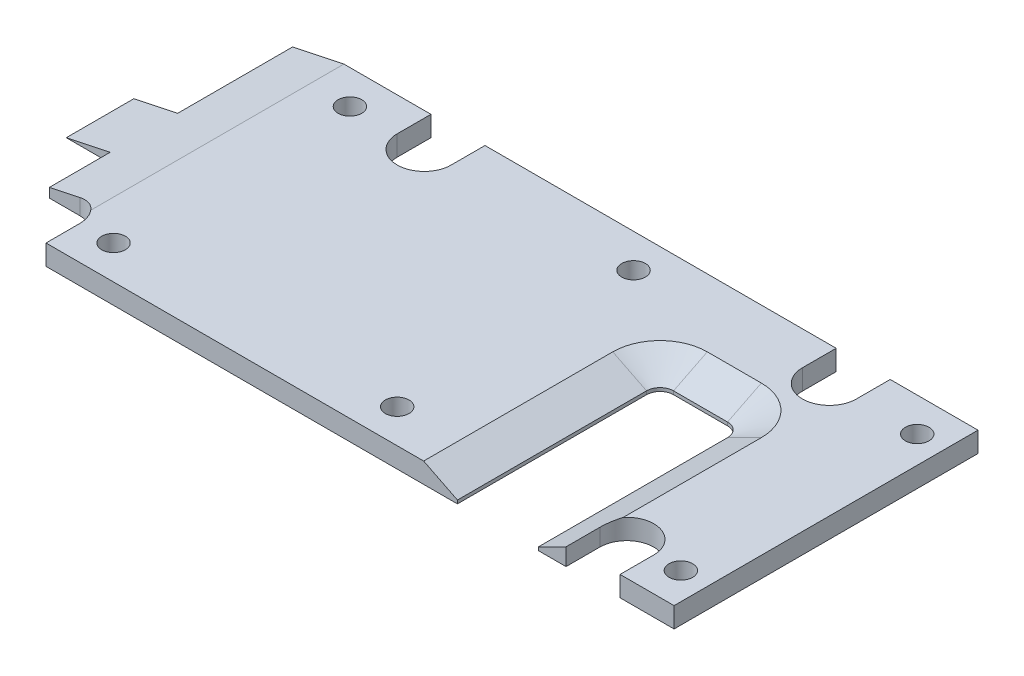
from build123d import *

# Parameters (mm, degrees)
SKETCH1_W           = 104.5
SKETCH1_H           = 45
BOSS_EXTRUDE1_DEPTH = 3
SKETCH2_W           = 12
SKETCH2_H           = 30
CUT_EXTRUDE1_DEPTH  = 34
SKETCH3_W           = 3
SKETCH3_H           = 45
CUT_EXTRUDE2_DEPTH  = 10
SKETCH4_R           = 1.75
CUT_EXTRUDE3_DEPTH  = 10
SKETCH5_W           = 10
SKETCH5_H           = 3
BOSS_EXTRUDE2_DEPTH = 6.5
CUT_EXTRUDE4_DEPTH  = 75.064583304
SKETCH7_R           = 4
CUT_EXTRUDE5_DEPTH  = 10
SKETCH8_W           = 8
SKETCH8_H           = 8.668176015
CUT_EXTRUDE6_DEPTH  = 10
FILLET1_R           = 2
CHAMFER2_SIZE       = 5
CHAMFER2_SIZE2      = 2.5


with BuildPart() as part:
    # Sketch1 → Boss-Extrude1 (new body)
    with BuildSketch(Plane(origin=(0, 0, 0), x_dir=(1, 0, 0), z_dir=(0, 1, 0))):
        Rectangle(SKETCH1_W, SKETCH1_H)
    extrude(amount=BOSS_EXTRUDE1_DEPTH)

    # Sketch2 → Cut-Extrude1 (cut)
    with BuildSketch(Plane(origin=(0, 3, 0), x_dir=(1, 0, 0), z_dir=(0, 1, 0))):
        with Locations((23.17, -7.5)):
            Rectangle(SKETCH2_W, SKETCH2_H)
    extrude(amount=-CUT_EXTRUDE1_DEPTH, mode=Mode.SUBTRACT)

    # Sketch3 → Cut-Extrude2 (cut)
    with BuildSketch(Plane(origin=(0, 3, 0), x_dir=(1, 0, 0), z_dir=(0, 1, 0))):
        with Locations((50.75, 0)):
            Rectangle(SKETCH3_W, SKETCH3_H)
    extrude(amount=-CUT_EXTRUDE2_DEPTH, mode=Mode.SUBTRACT)

    # Sketch4 → Cut-Extrude3 (cut)
    with BuildSketch(Plane(origin=(0, 3, 0), x_dir=(1, 0, 0), z_dir=(0, 1, 0))):
        with Locations(Location((45.25, 17.5, 0), (0, 0, 270))):
            Circle(SKETCH4_R)
        with Locations(Location((45.25, -17.5, 0), (0, 0, 270))):
            Circle(SKETCH4_R)
        with Locations(Location((-38.75, 17.5, 0), (0, 0, 270))):
            Circle(SKETCH4_R)
        with Locations(Location((3.25, 17.5, 0), (0, 0, 270))):
            Circle(SKETCH4_R)
        with Locations(Location((-38.75, -17.5, 0), (0, 0, 270))):
            Circle(SKETCH4_R)
        with Locations(Location((3.25, -17.5, 0), (0, 0, 270))):
            Circle(SKETCH4_R)
    extrude(amount=-CUT_EXTRUDE3_DEPTH, mode=Mode.SUBTRACT)

    # Sketch5 → Boss-Extrude2 (add)
    with BuildSketch(Plane.ZY.offset(52.25)):
        with Locations((-0.5, 1.5)):
            Rectangle(SKETCH5_W, SKETCH5_H)
    extrude(amount=BOSS_EXTRUDE2_DEPTH)

    # Sketch6 → Cut-Extrude4 (cut, through all)
    with BuildSketch(Plane.XY.offset(22.5)):
        Polygon((-58.75, 0), (-44.636109672, 3), (-58.75, 3), align=None)
    extrude(amount=-CUT_EXTRUDE4_DEPTH, mode=Mode.SUBTRACT)

    # Sketch7 → Cut-Extrude5 (cut)
    with BuildSketch(Plane(origin=(0, 3, 0), x_dir=(1, 0, 0), z_dir=(0, 1, 0))):
        with Locations(Location((-27.75, 17.5, 0), (0, 0, 270))):
            Circle(SKETCH7_R)
        with Locations(Location((-47.75, -17.5, 0), (0, 0, 270))):
            Circle(SKETCH7_R)
        with Locations(Location((32.25, 17.5, 0), (0, 0, 270))):
            Circle(SKETCH7_R)
        with Locations(Location((37.25, -17.5, 0), (0, 0, 270))):
            Circle(SKETCH7_R)
    extrude(amount=-CUT_EXTRUDE5_DEPTH, mode=Mode.SUBTRACT)

    # Sketch8 → Cut-Extrude6 (cut)
    with BuildSketch(Plane(origin=(0, 3, 0), x_dir=(1, 0, 0), z_dir=(0, 1, 0))):
        with Locations((-27.75, 21.834088008)):
            Rectangle(SKETCH8_W, SKETCH8_H)
        with Locations((32.25, 21.834088008)):
            Rectangle(SKETCH8_W, SKETCH8_H)
        with BuildLine():
            Line((41.25, -17.5), (41.25, -22.5))
            Line((41.25, -22.5), (33.25, -22.5))
            Line((33.25, -22.5), (33.25, -17.5))
            ThreePointArc((33.25, -17.5), (37.25, -13.5), (41.25, -17.5))
        make_face()
        with BuildLine():
            Line((-43.75, -17.5), (-43.75, -22.5))
            Line((-43.75, -22.5), (-52.25, -22.5))
            Line((-52.25, -22.5), (-52.25, -13.5))
            Line((-52.25, -13.5), (-47.75, -13.5))
            ThreePointArc((-47.75, -13.5), (-44.921572875, -14.671572875), (-43.75, -17.5))
        make_face()
    extrude(amount=-CUT_EXTRUDE6_DEPTH, mode=Mode.SUBTRACT)

    # Fillet1
    fillet1_edges = [part.edges().sort_by_distance(p)[0] for p in [
        (29.17, 1.5, -7.5),
        (17.17, 1.5, -7.5),
    ]]
    fillet(fillet1_edges, radius=FILLET1_R)

    # Chamfer2
    chamfer2_edges = [part.edges().sort_by_distance(p)[0] for p in [
        (29.17, 3, 8.5),
        (28.584213562, 3, -6.914213562),
        (23.17, 3, -7.5),
        (17.755786438, 3, -6.914213562),
        (17.17, 3, 8.5),
    ]]
    chamfer2_side = [part.faces().sort_by_distance(p)[0] for p in [
        (-0.332275855, 3, -0.451474159),
    ]]
    chamfer(chamfer2_edges, length=CHAMFER2_SIZE, length2=CHAMFER2_SIZE2, reference=chamfer2_side[0])


solid = part.part
